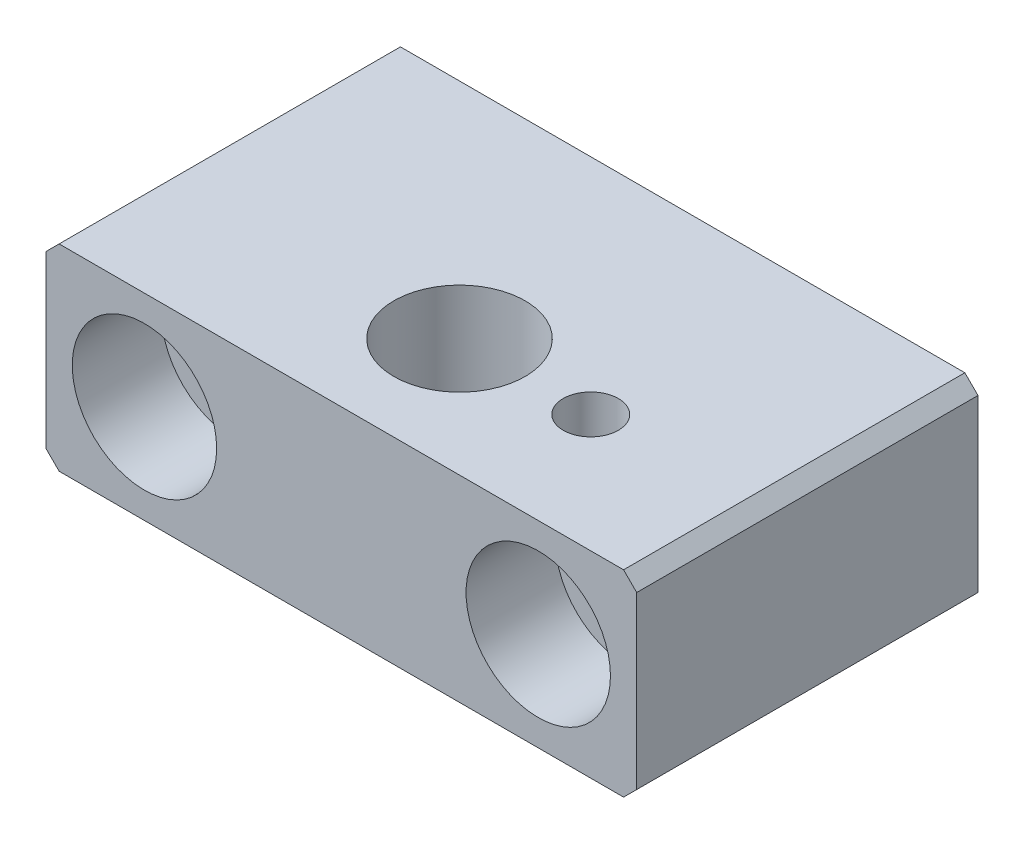
from build123d import *

# Parameters (mm, degrees)
SKETCH1_W                                            = 45
SKETCH1_H                                            = 26
BOSS_EXTRUDE1_DEPTH                                  = 15
SKETCH2_R                                            = 5
CUT_EXTRUDE1_DEPTH                                   = 31.004166377
F_6_0MM_DOWEL_HOLE_1_D                               = 6
F_6_0MM_DOWEL_HOLE_1_DEPTH                           = 10
F_6_0MM_DOWEL_HOLE_1_TIP                             = 1.802581857
CHAMFER1_SIZE                                        = 1
CBORE_FOR_M6_HEXAGON_SOCKET_HEAD_CAP_SCR_D           = 6.6
CBORE_FOR_M6_HEXAGON_SOCKET_HEAD_CAP_SCR_CBORE_D     = 11
CBORE_FOR_M6_HEXAGON_SOCKET_HEAD_CAP_SCR_CBORE_DEPTH = 6.8
M5_TAPPED_HOLE1_D                                    = 4.2
M5_TAPPED_HOLE1_DEPTH                                = 14
M5_TAPPED_HOLE1_TIP                                  = 1.2618073


with BuildPart() as part:
    # Sketch1 → Boss-Extrude1 (new body)
    with BuildSketch(Plane(origin=(0, 0, 0), x_dir=(1, 0, 0), z_dir=(0, 1, 0))):
        Rectangle(SKETCH1_W, SKETCH1_H)
    extrude(amount=BOSS_EXTRUDE1_DEPTH)

    # Sketch2 → Cut-Extrude1 (cut, through all)
    with BuildSketch(Plane(origin=(0, 15, 0), x_dir=(1, 0, 0), z_dir=(0, 1, 0))):
        with Locations(Location((0, -4, 0), (0, 0, 270))):
            Circle(SKETCH2_R)
    extrude(amount=-CUT_EXTRUDE1_DEPTH, mode=Mode.SUBTRACT)

    # Ø6.0mm Dowel Hole 1
    with Locations(Plane(origin=(0, 0, -13), x_dir=(-1, 0, 0), z_dir=(0, 0, -1))):
        with Locations((-5, 7.5), (5, 7.5)):
            Hole(F_6_0MM_DOWEL_HOLE_1_D / 2, depth=F_6_0MM_DOWEL_HOLE_1_DEPTH)
            with Locations((0, 0, -(F_6_0MM_DOWEL_HOLE_1_DEPTH + F_6_0MM_DOWEL_HOLE_1_TIP / 2))):  # 118° drill point
                Cone(0, F_6_0MM_DOWEL_HOLE_1_D / 2, F_6_0MM_DOWEL_HOLE_1_TIP, mode=Mode.SUBTRACT)

    # Chamfer1
    chamfer1_edges = [part.edges().sort_by_distance(p)[0] for p in [
        (-22.5, 15, 0),
        (22.5, 15, 0),
        (-22.5, 0, 0),
        (22.5, 0, 0),
    ]]
    chamfer(chamfer1_edges, length=CHAMFER1_SIZE)

    # CBORE for M6 Hexagon socket head cap screws1 (through all)
    with Locations(Plane.XY.offset(13)):
        with Locations((-15, 7.5), (15, 7.5)):
            CounterBoreHole(CBORE_FOR_M6_HEXAGON_SOCKET_HEAD_CAP_SCR_D / 2, CBORE_FOR_M6_HEXAGON_SOCKET_HEAD_CAP_SCR_CBORE_D / 2, CBORE_FOR_M6_HEXAGON_SOCKET_HEAD_CAP_SCR_CBORE_DEPTH)

    # M5 Tapped Hole1
    with Locations(Plane(origin=(0, 15, 0), x_dir=(1, 0, 0), z_dir=(0, 1, 0))):
        with Locations((10, -4)):
            Hole(M5_TAPPED_HOLE1_D / 2, depth=M5_TAPPED_HOLE1_DEPTH)
            with Locations((0, 0, -(M5_TAPPED_HOLE1_DEPTH + M5_TAPPED_HOLE1_TIP / 2))):  # 118° drill point
                Cone(0, M5_TAPPED_HOLE1_D / 2, M5_TAPPED_HOLE1_TIP, mode=Mode.SUBTRACT)


solid = part.part
